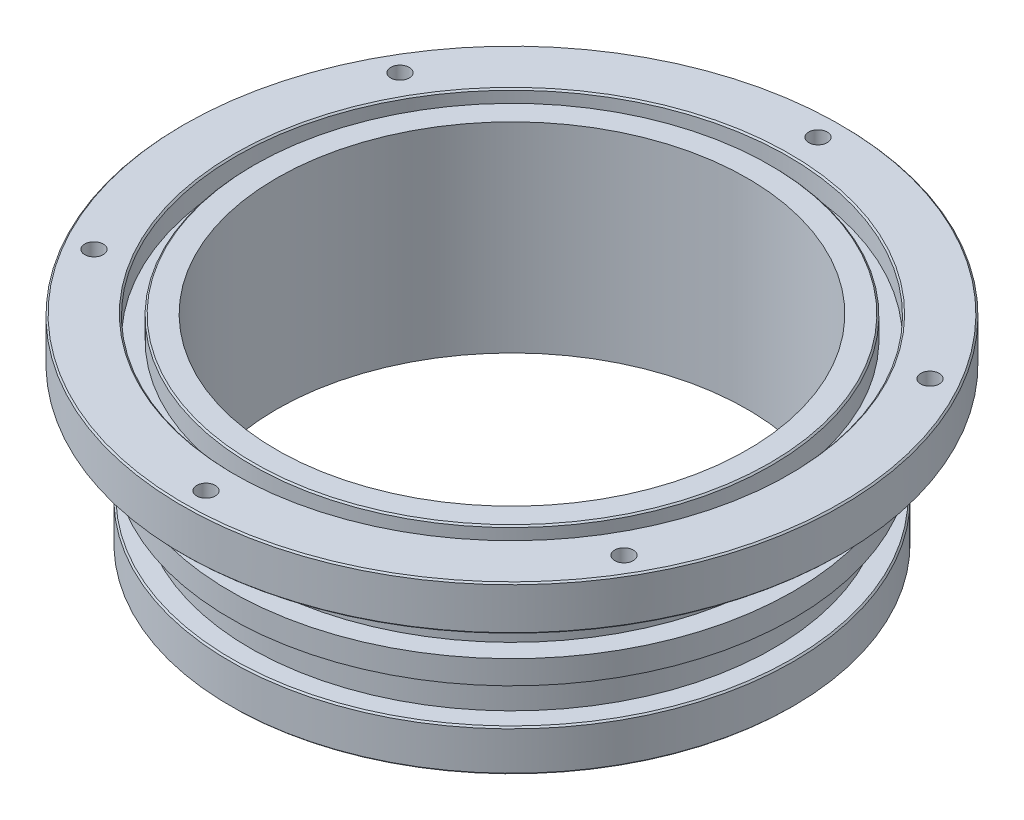
SolidWorks part; units mm, degrees
ref_plane "前视基准面" through (0, 0, 0) normal (0, 0, 1) x (1, 0, 0)
ref_plane "上视基准面" through (0, 0, 0) normal (0, 1, 0) x (1, 0, 0)
ref_plane "右视基准面" through (0, 0, 0) normal (1, 0, 0) x (0, 0, -1)
sketch "草图1" plane through (0, 0, 0) normal (0, 0, 1) x (1, 0, 0)
  line L0 (0, 27) -> (0, 0) construction
  line L1 (-31.75, 27) -> (-31.75, 0)
  line L2 (-31.75, 0) -> (-37.973, 0)
  line L3 (-37.973, 21) -> (-37.973, 18.413)
  line L4 (-35.2806, 5.587) -> (-37.973, 5.587)
  line L5 (-35.2806, 5.587) -> (-35.2806, 10.413)
  line L6 (-35.2806, 10.413) -> (-37.973, 10.413)
  line L7 (-35.2806, 13.587) -> (-37.973, 13.587)
  line L8 (-35.2806, 13.587) -> (-35.2806, 18.413)
  line L9 (-35.2806, 18.413) -> (-37.973, 18.413)
  line L10 (-37.973, 21) -> (-44.45, 21)
  line L11 (-44.45, 21) -> (-44.45, 27)
  line L12 (-44.45, 27) -> (-31.75, 27)
  line L13 (-37.973, 13.587) -> (-37.973, 10.413)
  line L14 (-37.973, 5.587) -> (-37.973, 0)
revolve "旋转1" add sketch "草图1" angle 360 about L0
chamfer "倒角1" distance 0.2 angle 45 4 edges at (-37.973, 5.587, 0) (-37.973, 0, 0) (-44.45, 27, 0) (-44.45, 21, 0)
hole_wizard "M3 螺纹孔1" positions "草图2" profile "草图3" tap size "M3" standard "GB"
sketch "草图2" plane through (0, 27, 0) normal (0, 1, 0) x (1, 0, 0)
  point P3 (-35.7452, -20.6375)
  point P4 (-35.7452, 20.6375)
  point P6 (0, 41.275)
  point P7 (35.7452, 20.6375)
  point P8 (35.7452, -20.6375)
  point P9 (0, -41.275)
sketch "草图3" plane through (-35.7452, 27, 20.6375) normal (1, 0, 0) x (0, 0, 1)
  line L0 (0, 0) -> (0, 8.2511)
  line L1 (0, 8.2511) -> (1.25, 7.5)
  line L2 (1.25, 7.5) -> (1.25, 0)
  line L5 (1.25, 0) -> (0, 0)
  line L10 (0, 8.2511) -> (-1.25, 7.5) construction
  line L11 (0, -6.35) -> (0, 107.95) construction
  dimension "螺纹孔钻头直径" = 2.5
  dimension "螺纹孔钻头深度" = 7.5
  dimension "导头角度" = 118
cosmetic thread "孔螺蚊线1" parameters "D1"=6, "D2"=3
cosmetic thread "孔螺蚊线2" parameters "D1"=6, "D2"=3
cosmetic thread "孔螺蚊线3" parameters "D1"=6, "D2"=3
cosmetic thread "孔螺蚊线4" parameters "D1"=6, "D2"=3
cosmetic thread "孔螺蚊线5" parameters "D1"=6, "D2"=3
cosmetic thread "孔螺蚊线6" parameters "D1"=6, "D2"=3
sketch "草图4" plane through (0, 27, 0) normal (0, 1, 0) x (1, 0, 0)
  circle A0 centre (0, 0) radius 35
  circle A1 centre (0, 0) radius 37.25
  dimension "D1" = 70
  dimension "D2" = 74.5
extrude "切除-拉伸1" cut sketch "草图4" against normal blind 3
chamfer "倒角2" distance 0.2 angle 45 2 edges at (-37.25, 27, 0) (-35, 27, 0)
